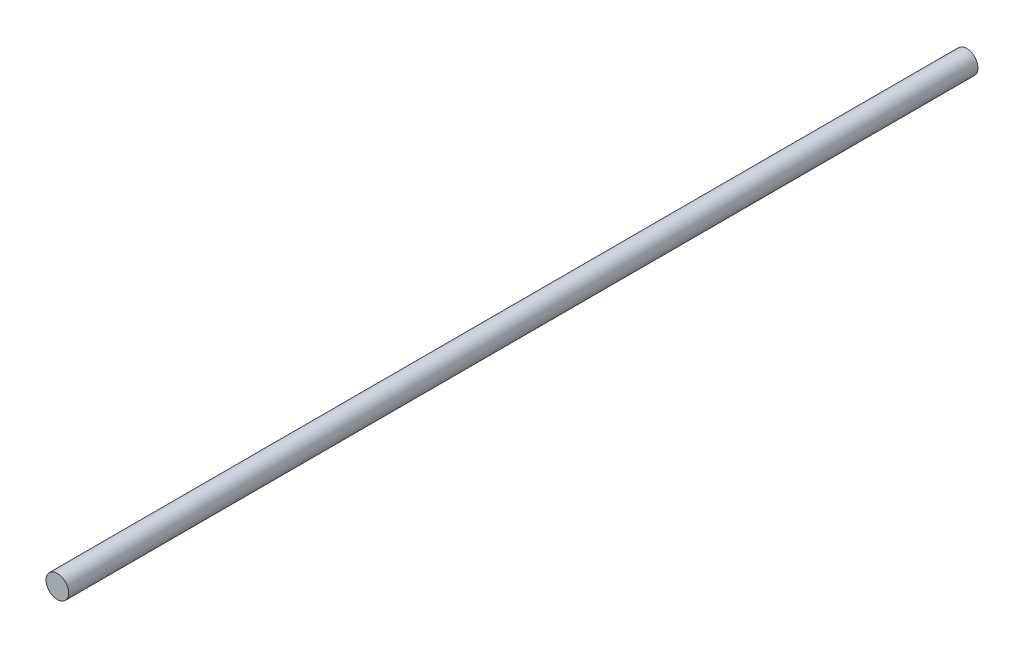
from build123d import *

# Parameters (mm, degrees)
SKETCH_1_R      = 5
EXTRUDE_1_DEPTH = 400


with BuildPart() as part:
    # 草图1 → 凸台-拉伸1 (new body)
    with BuildSketch(Plane.XY):
        Circle(SKETCH_1_R)
    extrude(amount=EXTRUDE_1_DEPTH)


solid = part.part
